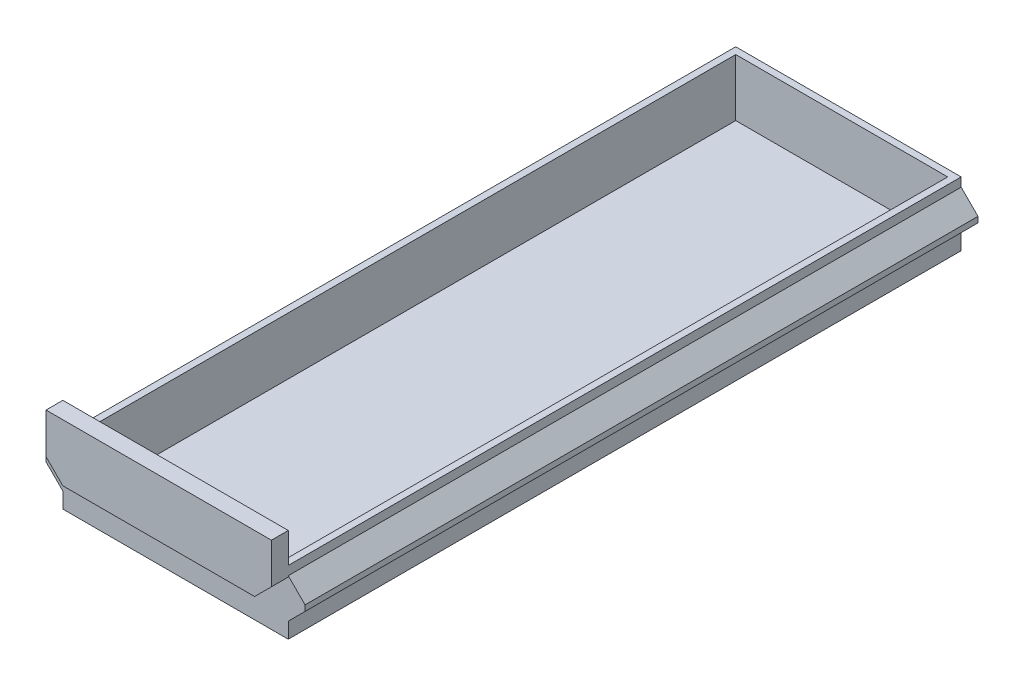
SolidWorks part; units mm, degrees
ref_plane "Front Plane" through (0, 0, 0) normal (0, 0, 1) x (1, 0, 0)
ref_plane "Top Plane" through (0, 0, 0) normal (0, 1, 0) x (1, 0, 0)
ref_plane "Right Plane" through (0, 0, 0) normal (1, 0, 0) x (0, 0, -1)
sketch "Sketch1" plane through (0, 0, 0) normal (0, 0, 1) x (1, 0, 0)
  line L0 (-73, 28) -> (-6, 28)
  line L1 (-73, 28) -> (-73, 32.6569)
  line L2 (-73, 32.6569) -> (-78, 37.6569)
  line L3 (-78, 37.6569) -> (-78, 39.3532)
  line L4 (-78, 39.3532) -> (-73, 44.3532)
  line L5 (-73, 44.3532) -> (-73, 47)
  line L6 (77, 47) -> (74, 47) construction
  line L7 (-73, 47) -> (-6, 47)
  line L8 (-39.5, 47) -> (-39.5, 28) construction
  line L9 (-83, 37) -> (-77, 31) construction
  line L10 (-77, 47) -> (-83, 41) construction
  line L11 (-83, 41) -> (-83, 37) construction
  line L12 (-74, 18) -> (-74, 23) construction
  line L13 (-6, 44.3532) -> (-6, 47)
  line L14 (-1, 39.3532) -> (-6, 44.3532)
  line L15 (-1, 37.6569) -> (-1, 39.3532)
  line L16 (-6, 32.6569) -> (-1, 37.6569)
  line L17 (-6, 28) -> (-6, 32.6569)
  dimension "D1" = 19
  dimension "D2" = 4
  dimension "D3" = 5
  dimension "D4" = 4.7
  dimension "D5" = 1
  dimension "D6" = 77
extrude "Boss-Extrude1" add sketch "Sketch1" against normal blind 200
sketch "Sketch2" plane through (0, 47, 0) normal (0, 1, 0) x (1, 0, 0)
  line L8 (-71, 2) -> (-8, 2)
  line L9 (-8, 2) -> (-8, 198)
  line L10 (-8, 198) -> (-71, 198)
  line L11 (-71, 198) -> (-71, 2)
  line L12 (-71, 2) -> (-8, 2)
  line L13 (-8, 2) -> (-8, 198)
  line L14 (-8, 198) -> (-71, 198)
  line L15 (-71, 198) -> (-71, 2)
  dimension "D1" = 2
extrude "Cut-Extrude1" cut sketch "Sketch2" against normal offset from surface (17 mm away) 2 up to face at (-39.5, 28, -100)
sketch "Sketch3" plane through (0, 0, 0) normal (0, 0, 1) x (1, 0, 0)
  line L0 (-73, 47) -> (-73, 44.3532) construction
  line L1 (-73, 56) -> (-6, 56)
  line L2 (-73, 56) -> (-73, 39)
  line L3 (-73, 39) -> (-6, 39)
  line L4 (-6, 56) -> (-6, 39)
  line L6 (-6, 44.3532) -> (-6, 47) construction
  line L7 (87.5, 56) -> (-87.5, 56) construction
  line L8 (-6, 47) -> (-73, 47) construction
  dimension "D1" = 8
extrude "Boss-Extrude2" add sketch "Sketch3" along normal blind 5
chamfer "Chamfer1" distance 5 angle 45 2 edges at (-73, 39, 2.5) (-6, 39, 2.5)
